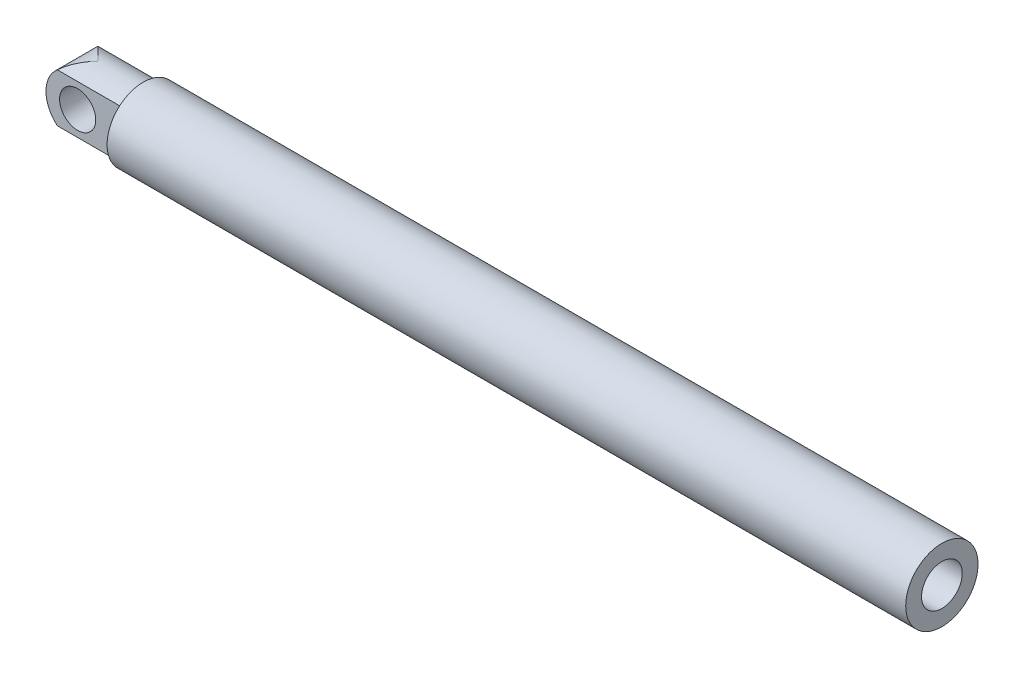
SolidWorks part; units mm, degrees
ref_plane "Front Plane" through (0, 0, 0) normal (0, 0, 1) x (1, 0, 0)
ref_plane "Top Plane" through (0, 0, 0) normal (0, 1, 0) x (1, 0, 0)
ref_plane "Right Plane" through (0, 0, 0) normal (1, 0, 0) x (0, 0, -1)
sketch "Sketch 1" plane through (0, 0, 0) normal (0, 0, 1) x (1, 0, 0)
  line L0 (0, 98.1295) -> (0, -117.1223) construction
  line L1 (-802.1676, 0) -> (65.6115, 0) construction
  line L3 (0, 40) -> (-883, 40)
  line L4 (-883, 40) -> (-883, 35)
  line L5 (-883, 35) -> (-968, 35)
  line L6 (-968, 35) -> (-968, 0)
  line L8 (0, 22.5) -> (-750, 22.5)
  line L9 (-750, 22.5) -> (-750, 0)
  line L10 (0, 40) -> (0, 22.5)
  line L11 (-968, 0) -> (-750, 0)
  dimension "D1" = 80
  dimension "D2" = 70
  dimension "D3" = 85
  dimension "D4" = 968
  dimension "D5" = 45
  dimension "D6" = 218
revolve "Revolve 1" add sketch "Sketch 1" angle 360 about L1
sketch "Sketch 2" plane through (0, 0, 0) normal (0, 0, 1) x (1, 0, 0)
  line L0 (-707.9802, 0) -> (-446.4102, 0) construction
  line L2 (-968, -35) -> (-968, 35)
  line L3 (-968, 35) -> (-933, 35)
  line L5 (-883, 35) -> (-968, 35) construction
  line L6 (-968, -35) -> (-933, -35)
  arc A0 (-933, 35) -> (-933, -35) centre (-933, 0) ccw
  circle A1 centre (-933, 0) radius 20
  point P13 (-968, 0)
  dimension "D1" = 40
extrude "Cut-Extrude 1" cut sketch "Sketch 2" against normal through all both and the other way through all contours A1 L0 | L0 A1 | A0 L3 L2 | A0 L2 L6
sketch "Sketch 3" plane through (-883, 0, 0) normal (-1, 0, 0) x (0, 0, 1)
  line L0 (0, 52.973) -> (0, -56.0607) construction
  line L1 (-82.2095, 0) -> (76.6131, 0) construction
  line L2 (-22.5, 50) -> (-50.6751, 50)
  line L3 (-22.5, 50) -> (-22.5, -50)
  line L4 (-22.5, -50) -> (-50.6751, -50)
  line L5 (-50.6751, 50) -> (-50.6751, -50)
  line L6 (50.6751, 50) -> (50.6751, -50)
  line L7 (22.5, -50) -> (50.6751, -50)
  line L8 (22.5, 50) -> (22.5, -50)
  line L9 (22.5, 50) -> (50.6751, 50)
  dimension "D1" = 45
  dimension "D2" = 100
  dimension "D3" = 28.1751
extrude "Cut-Extrude 2" cut sketch "Sketch 3" along normal through all
